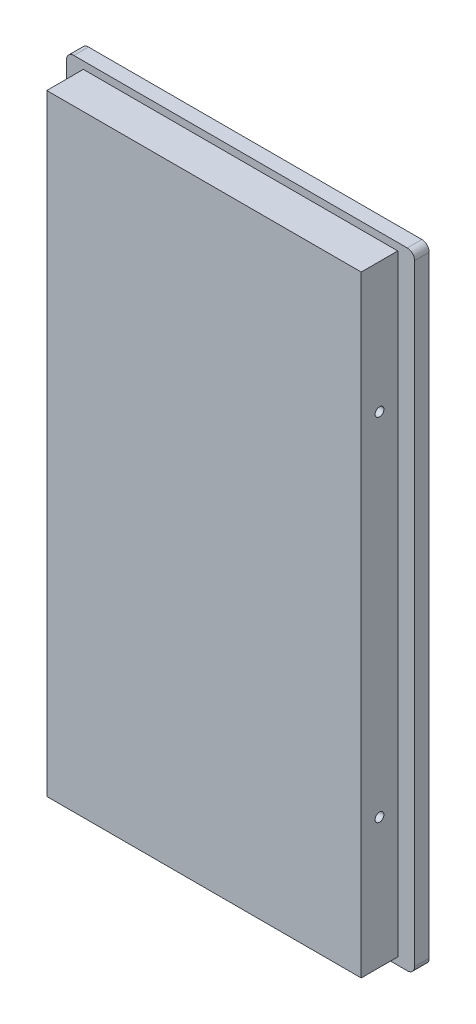
SolidWorks part; units mm, degrees
ref_plane "前视基准面" through (0, 0, 0) normal (0, 0, 1) x (1, 0, 0)
ref_plane "上视基准面" through (0, 0, 0) normal (0, 1, 0) x (1, 0, 0)
ref_plane "右视基准面" through (0, 0, 0) normal (1, 0, 0) x (0, 0, -1)
sketch "草图1" plane through (0, 0, 0) normal (0, 0, 1) x (1, 0, 0)
  line L1 (-114, 214) -> (114, 214)
  line L2 (-119, 209) -> (-119, -209)
  line L3 (-114, -214) -> (114, -214)
  line L4 (119, 209) -> (119, -209)
  line L5 (-119, 214) -> (119, -214) construction
  line L6 (-119, -214) -> (119, 214) construction
  arc A0 (-119, -209) -> (-114, -214) centre (-114, -209) ccw
  arc A1 (119, -209) -> (114, -214) centre (114, -209) cw
  arc A2 (119, 209) -> (114, 214) centre (114, 209) ccw
  arc A3 (-119, 209) -> (-114, 214) centre (-114, 209) cw
  point P0 (0, 0)
  dimension "D3" = 5
  dimension "D1" = 238
  dimension "D2" = 428
extrude "凸台-拉伸1" add sketch "草图1" along normal blind 10
sketch "草图2" plane through (0, 0, 10) normal (0, 0, 1) x (1, 0, 0)
  line L1 (-107.5, 209) -> (107.5, 209)
  line L2 (-107.5, 209) -> (-107.5, -209)
  line L3 (-107.5, -209) -> (107.5, -209)
  line L4 (107.5, 209) -> (107.5, -209)
  line L5 (-107.5, 209) -> (107.5, -209) construction
  line L6 (-107.5, -209) -> (107.5, 209) construction
  point P0 (0, 0)
  dimension "D1" = 215
  dimension "D2" = 418
extrude "凸台-拉伸2" add sketch "草图2" along normal blind 25
sketch "草图3" plane through (107.5, 0, 0) normal (1, 0, 0) x (0, 0, -1)
  line L0 (-10, 0) -> (-88.8821, 0) construction
  line L1 (-10, -209) -> (-10, 209) construction
  line L2 (-35, -209) -> (-35, 209) construction
  circle A0 centre (-22.5, 120) radius 3
  circle A1 centre (-22.5, -120) radius 3
  dimension "D1" = 12.5
  dimension "D2" = 240
  dimension "D3" = 6
extrude "切除-拉伸1" cut sketch "草图3" against normal through all both and the other way through all
sketch "草图4" plane through (0, 0, 0) normal (0, 0, -1) x (-1, 0, 0)
  line L0 (0, 214) -> (0, -214) construction
  line L1 (-114, 214) -> (114, 214) construction
  line L2 (114, -214) -> (-114, -214) construction
  line L3 (-12.5, 34) -> (12.5, 34) construction
  line L4 (-50, 164) -> (50, 164)
  line L5 (-50, 164) -> (-50, 104)
  line L6 (-50, 104) -> (50, 104)
  line L7 (50, 164) -> (50, 104)
  line L8 (-50, 164) -> (50, 104) construction
  line L9 (-50, 104) -> (50, 164) construction
  line L10 (-12.5, 36) -> (12.5, 36)
  line L11 (-12.5, 32) -> (12.5, 32)
  line L12 (27.5, 34) -> (52.5, 34) construction
  line L13 (27.5, 36) -> (52.5, 36)
  line L14 (27.5, 32) -> (52.5, 32)
  line L15 (-27.5, 34) -> (-52.5, 34) construction
  line L16 (-27.5, 36) -> (-52.5, 36)
  line L17 (-27.5, 32) -> (-52.5, 32)
  line L18 (0, -26) -> (60, -26) construction
  arc A0 (-12.5, 36) -> (-12.5, 32) centre (-12.5, 34) ccw
  arc A1 (12.5, 32) -> (12.5, 36) centre (12.5, 34) ccw
  arc A2 (27.5, 36) -> (27.5, 32) centre (27.5, 34) ccw
  arc A3 (52.5, 32) -> (52.5, 36) centre (52.5, 34) ccw
  arc A4 (-27.5, 36) -> (-27.5, 32) centre (-27.5, 34) cw
  arc A5 (-52.5, 32) -> (-52.5, 36) centre (-52.5, 34) cw
  circle A6 centre (0, -26) radius 12.5
  circle A7 centre (60, -26) radius 12.5
  circle A8 centre (60, -86) radius 12.5
  circle A9 centre (60, -146) radius 12.5
  circle A10 centre (0, -86) radius 12.5
  circle A11 centre (0, -146) radius 12.5
  circle A12 centre (-60, -146) radius 12.5
  circle A13 centre (-60, -86) radius 12.5
  circle A14 centre (-60, -26) radius 12.5
  point P6 (0, 134)
  point P13 (0, 34)
  point P19 (40, 34)
  point P27 (-40, 34)
  dimension "D1" = 2
  dimension "D7" = 2
  dimension "D10" = 25
  dimension "D15" = 60
  dimension "D2" = 60
  dimension "D3" = 100
  dimension "D4" = 80
  dimension "D5" = 25
  dimension "D6" = 100
  dimension "D8" = 25
  dimension "D9" = 40
  dimension "D11" = 60
  dimension "D14" = 60
  dimension "D12" = 2
  dimension "D13" = 3
extrude "切除-拉伸2" cut sketch "草图4" against normal blind 1
move or copy body "实体-移动/复制1" [suppressed] bodies to move or copy 104
